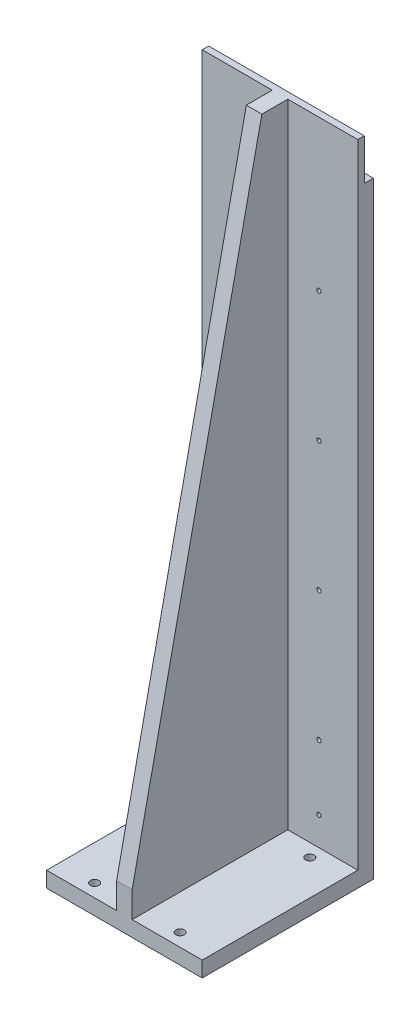
from build123d import *

# Parameters (mm, degrees)
SKETCH1_W                = 120
SKETCH1_H                = 500
BOSS_EXTRUDE1_DEPTH      = 12
SKETCH2_W                = 120
SKETCH2_H                = 12
BOSS_EXTRUDE2_DEPTH      = 120
BOSS_EXTRUDE3_DEPTH      = 6
M6_CLEARANCE_HOLE1_D     = 6.6
M6_CLEARANCE_HOLE1_DEPTH = 15
M6_CLEARANCE_HOLE1_TIP   = 1.982840043
M6_CLEARANCE_HOLE2_D     = 6.6
M6_CLEARANCE_HOLE2_DEPTH = 15
M6_CLEARANCE_HOLE2_TIP   = 1.982840043
M4_TAPPED_HOLE1_D        = 3.3
CUT_EXTRUDE1_DEPTH       = 308.122125546
CUT_EXTRUDE1_DEPTH_BACK  = 308.122125546
SKETCH10_W               = 7
SKETCH10_H               = 31.8


with BuildPart() as part:
    # Sketch1 → Boss-Extrude1 (new body)
    with BuildSketch(Plane.XY):
        Rectangle(SKETCH1_W, SKETCH1_H)
    extrude(amount=BOSS_EXTRUDE1_DEPTH)

    # Sketch2 → Boss-Extrude2 (add)
    with BuildSketch(Plane.XY.offset(12)):
        with Locations((0, -244)):
            Rectangle(SKETCH2_W, SKETCH2_H)
    extrude(amount=BOSS_EXTRUDE2_DEPTH)

    # Sketch3 → Boss-Extrude3 (add, symmetric)
    with BuildSketch(Plane(origin=(0, 0, 0), x_dir=(0, 0, -1), z_dir=(1, 0, 0))):
        Polygon((-12, 250), (-32, 250), (-132, -218), (-132, -238), (-12, -238), align=None)
    extrude(amount=BOSS_EXTRUDE3_DEPTH, both=True)

    # M6 Clearance Hole1
    with Locations(Plane(origin=(0, -238, 0), x_dir=(1, 0, 0), z_dir=(0, 1, 0))):
        with Locations((33, -122), (33, -22)):
            Hole(M6_CLEARANCE_HOLE1_D / 2, depth=M6_CLEARANCE_HOLE1_DEPTH)
            with Locations((0, 0, -(M6_CLEARANCE_HOLE1_DEPTH + M6_CLEARANCE_HOLE1_TIP / 2))):  # 118° drill point
                Cone(0, M6_CLEARANCE_HOLE1_D / 2, M6_CLEARANCE_HOLE1_TIP, mode=Mode.SUBTRACT)

    # M6 Clearance Hole2
    with Locations(Plane(origin=(0, -238, 0), x_dir=(1, 0, 0), z_dir=(0, 1, 0))):
        with Locations((-33, -122), (-33, -22)):
            Hole(M6_CLEARANCE_HOLE2_D / 2, depth=M6_CLEARANCE_HOLE2_DEPTH)
            with Locations((0, 0, -(M6_CLEARANCE_HOLE2_DEPTH + M6_CLEARANCE_HOLE2_TIP / 2))):  # 118° drill point
                Cone(0, M6_CLEARANCE_HOLE2_D / 2, M6_CLEARANCE_HOLE2_TIP, mode=Mode.SUBTRACT)

    # M4 Tapped Hole1 (through all)
    with Locations(Plane(origin=(0, 0, 0), x_dir=(-1, 0, 0), z_dir=(0, 0, -1))):
        with Locations((-30, 34), (-30, 134), (-30, -66), (-30, -166), (-30, -216), (30, -216), (30, -166), (30, -66), (30, 34), (30, 134)):
            Hole(M4_TAPPED_HOLE1_D / 2)

    # Sketch10 → Cut-Extrude1 (cut, two sides: drawn at the far end of the back side and taken through both)
    with BuildSketch(Plane(origin=(60, 0, 0), x_dir=(0, 0, -1), z_dir=(1, 0, 0)).offset(-CUT_EXTRUDE1_DEPTH_BACK)):
        with Locations((-3.5, 234.1)):
            Rectangle(SKETCH10_W, SKETCH10_H)
    extrude(amount=CUT_EXTRUDE1_DEPTH + CUT_EXTRUDE1_DEPTH_BACK, mode=Mode.SUBTRACT)


solid = part.part
